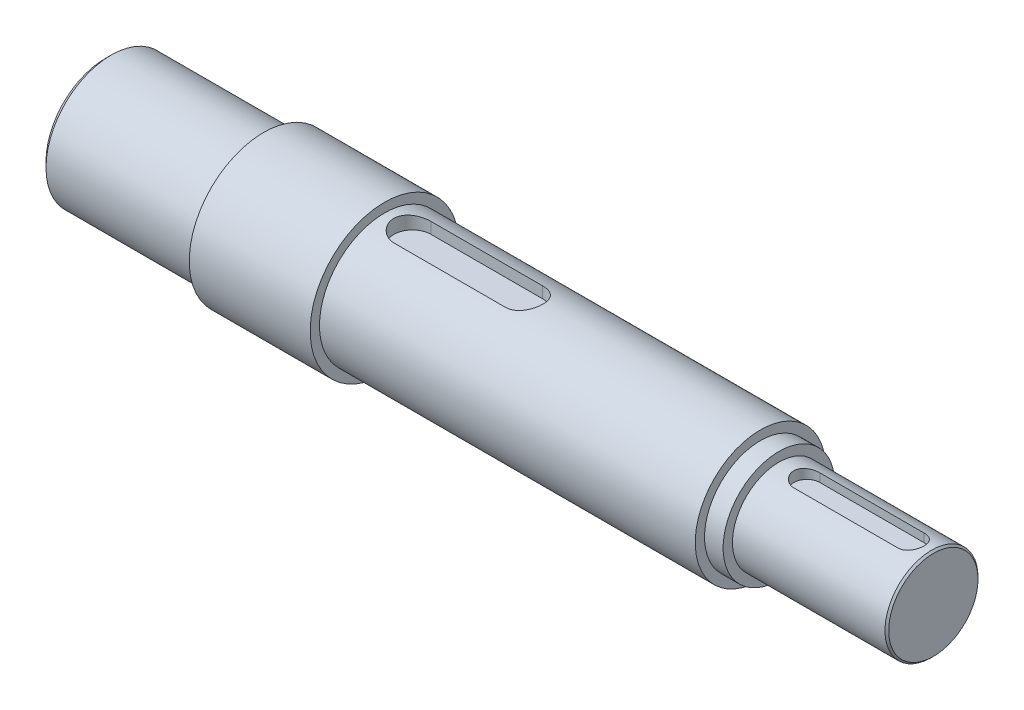
from build123d import *

# Parameters (mm, degrees)
SKETCH1_R      = 40
EXTRUDE1_DEPTH = 65
SKETCH2_R      = 35
EXTRUDE2_DEPTH = 202
EXTRUDE3_START = 85
SKETCH3_R      = 35
EXTRUDE3_DEPTH = 85
CHAMFER1_SIZE  = 3
EXTRUDE4_DEPTH = 7.5
SKETCH5_R      = 30
EXTRUDE5_DEPTH = 10
SKETCH7_R      = 25
EXTRUDE6_DEPTH = 83
EXTRUDE7_DEPTH = 10
CHAMFER2_SIZE  = 1


with BuildPart() as part:
    # Sketch1 → Extrude1 (new body)
    with BuildSketch(Plane(origin=(0, 0, 0), x_dir=(0, 0, -1), z_dir=(1, 0, 0))):
        Circle(SKETCH1_R)
    extrude(amount=EXTRUDE1_DEPTH)

    # Sketch2 → Extrude2 (add)
    with BuildSketch(Plane(origin=(65, 0, 0), x_dir=(0, 0, -1), z_dir=(1, 0, 0))):
        Circle(SKETCH2_R)
    extrude(amount=EXTRUDE2_DEPTH)

    # Sketch3 → Extrude3 (add)
    with BuildSketch(Plane.ZY.offset(EXTRUDE3_START)):
        with Locations(Location((0, 0, 0), (0, 0, 180))):
            Circle(SKETCH3_R)
    extrude(amount=-EXTRUDE3_DEPTH)

    # Chamfer1
    chamfer1_edges = [part.edges().sort_by_distance(p)[0] for p in [
        (-85, 0, 35),
    ]]
    chamfer(chamfer1_edges, length=CHAMFER1_SIZE)

    # Sketch4 → Extrude4 (cut)
    with BuildSketch(Plane(origin=(0, 27.5, 0), x_dir=(-1, 0, 0), z_dir=(0, 1, 0))):
        with BuildLine():
            Line((-80, 10), (-140, 10))
            ThreePointArc((-140, 10), (-150, 0), (-140, -10))
            Line((-140, -10), (-80, -10))
            ThreePointArc((-80, -10), (-70, 0), (-80, 10))
        make_face()
    extrude(amount=EXTRUDE4_DEPTH, mode=Mode.SUBTRACT)

    # Sketch5 → Extrude5 (add)
    with BuildSketch(Plane(origin=(267, 0, 0), x_dir=(0, 0, -1), z_dir=(1, 0, 0))):
        Circle(SKETCH5_R)
    extrude(amount=EXTRUDE5_DEPTH)

    # Sketch7 → Extrude6 (add)
    with BuildSketch(Plane(origin=(277, 0, 0), x_dir=(0, 0, -1), z_dir=(1, 0, 0))):
        Circle(SKETCH7_R)
    extrude(amount=EXTRUDE6_DEPTH)

    # Sketch8 → Extrude7 (cut)
    with BuildSketch(Plane(origin=(0, 19.5, 0), x_dir=(-1, 0, 0), z_dir=(0, 1, 0))):
        with BuildLine():
            Line((-292, 7), (-348, 7))
            ThreePointArc((-348, 7), (-355, 0), (-348, -7))
            Line((-348, -7), (-292, -7))
            ThreePointArc((-292, -7), (-285, 0), (-292, 7))
        make_face()
    extrude(amount=EXTRUDE7_DEPTH, mode=Mode.SUBTRACT)

    # Chamfer2
    chamfer2_edges = [part.edges().sort_by_distance(p)[0] for p in [
        (360, 0, 25),
    ]]
    chamfer(chamfer2_edges, length=CHAMFER2_SIZE)


solid = part.part
